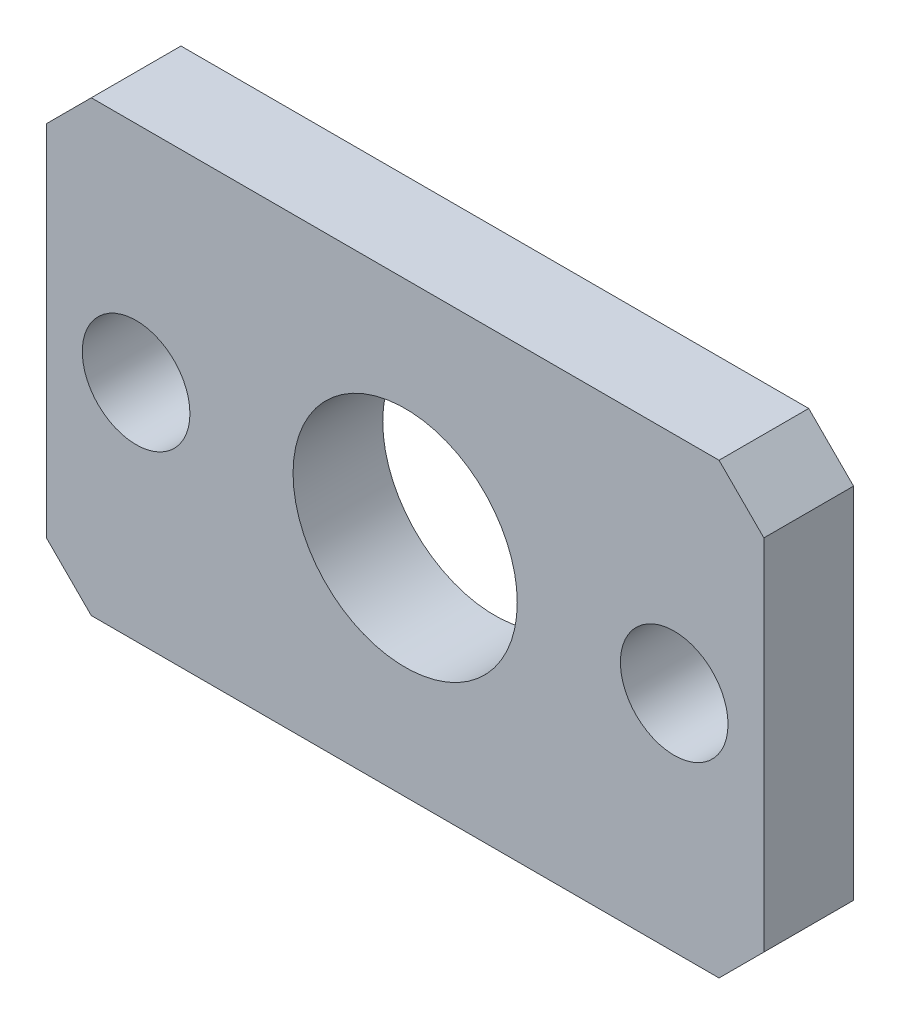
SolidWorks part; units mm, degrees
ref_plane "Front Plane" through (0, 0, 0) normal (0, 0, 1) x (1, 0, 0)
ref_plane "Top Plane" through (0, 0, 0) normal (0, 1, 0) x (1, 0, 0)
ref_plane "Right Plane" through (0, 0, 0) normal (1, 0, 0) x (0, 0, -1)
sketch "Sketch1" plane through (0, 0, 0) normal (0, 0, 1) x (1, 0, 0)
  line L1 (-4, 2.5) -> (4, 2.5)
  line L2 (-4, 2.5) -> (-4, -2.5)
  line L3 (-4, -2.5) -> (4, -2.5)
  line L4 (4, 2.5) -> (4, -2.5)
  line L5 (-4, 2.5) -> (4, -2.5) construction
  line L6 (-4, -2.5) -> (4, 2.5) construction
  point P0 (0, 0)
  dimension "D1" = 8
  dimension "D2" = 5
extrude "Boss-Extrude1" add sketch "Sketch1" along normal mid plane 1
sketch "Sketch2" plane through (0, 0, 0.5) normal (0, 0, 1) x (1, 0, 0)
  circle A0 centre (0, 0) radius 1.25
  circle A1 centre (-3, 0) radius 0.6
  circle A2 centre (3, 0) radius 0.6
  dimension "D1" = 2.5
  dimension "D2" = 1.2
  dimension "D6" = 3
  dimension "D3" = 6
extrude "Cut-Extrude1" cut sketch "Sketch2" against normal through all
chamfer "Chamfer1" distance 0.5 angle 45 4 edges at (-4, -2.5, 0) (-4, 2.5, 0) (4, -2.5, 0) (4, 2.5, 0)
